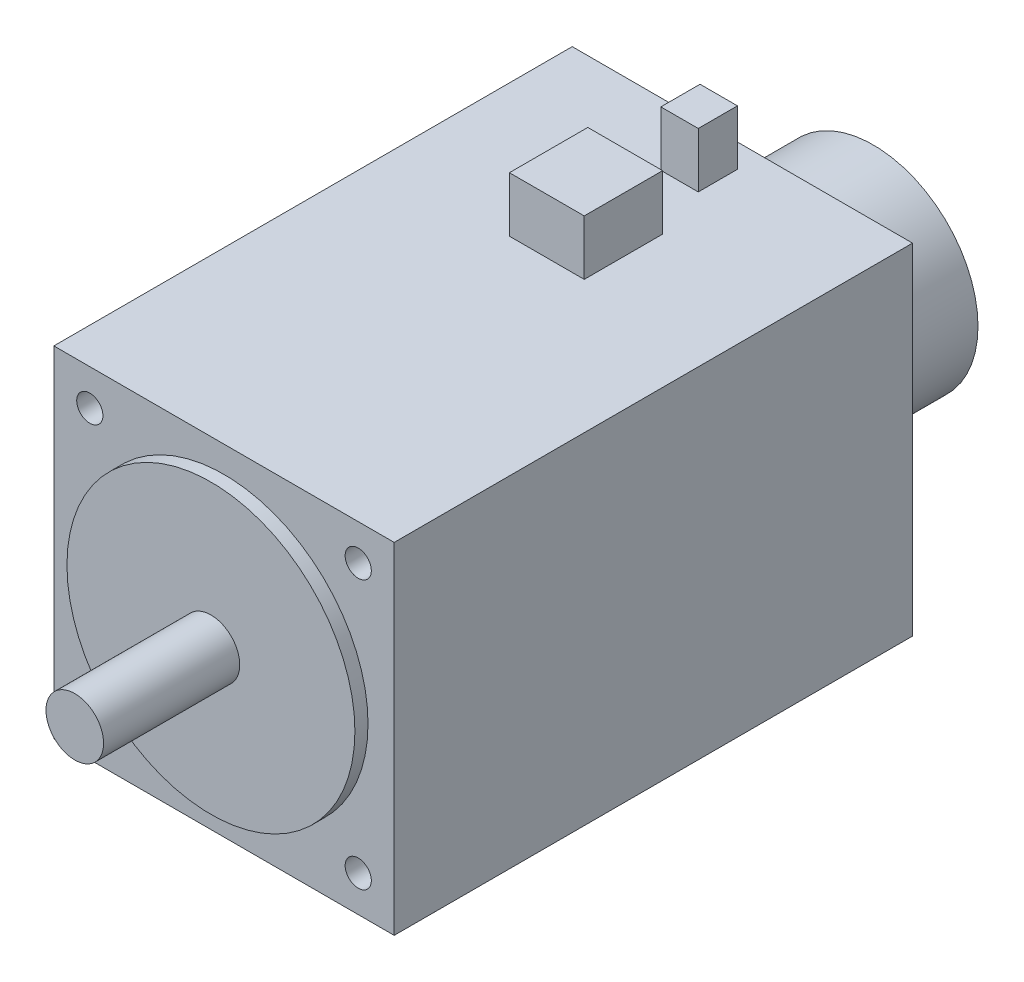
from build123d import *

# Parameters (mm, degrees)
SKETCH_1_W      = 130
SKETCH_1_H      = 130
SKETCH_1_R      = 5
EXTRUDE_1_DEPTH = 99
SKETCH_2_R      = 55
EXTRUDE_2_DEPTH = 5
SKETCH_3_R      = 11
EXTRUDE_3_DEPTH = 52
SKETCH_5_W      = 28.58431815
SKETCH_5_H      = 29.945476157
SKETCH_5_W_2    = 14.292159074
SKETCH_5_H_2    = 14.972738078
EXTRUDE_4_DEPTH = 86
SKETCH_6_R      = 40
EXTRUDE_5_DEPTH = 50


with BuildPart() as part:
    # 草图1 → 凸台-拉伸1 (new, symmetric)
    with BuildSketch(Plane.XY):
        Rectangle(SKETCH_1_W, SKETCH_1_H)
        with Locations((-51.265241636, 51.265241636)):
            Circle(SKETCH_1_R, mode=Mode.SUBTRACT)
        with Locations(Location((51.265241636, 51.265241636, 0), (0, 0, 180))):
            Circle(SKETCH_1_R, mode=Mode.SUBTRACT)
        with Locations(Location((-51.265241636, -51.265241636, 0), (0, 0, 180))):
            Circle(SKETCH_1_R, mode=Mode.SUBTRACT)
        with Locations((51.265241636, -51.265241636)):
            Circle(SKETCH_1_R, mode=Mode.SUBTRACT)
    extrude(amount=EXTRUDE_1_DEPTH, both=True)

    # 草图2 → 凸台-拉伸2 (add)
    with BuildSketch(Plane.XY.offset(99)):
        Circle(SKETCH_2_R)
    extrude(amount=EXTRUDE_2_DEPTH)

    # 草图3 → 凸台-拉伸3 (add)
    with BuildSketch(Plane.XY.offset(104)):
        with Locations(Location((0, 0, 0), (0, 0, 180))):
            Circle(SKETCH_3_R)
    extrude(amount=EXTRUDE_3_DEPTH)

    # 草图5 → 凸台-拉伸4 (add)
    with BuildSketch(Plane(origin=(0, 0, 0), x_dir=(1, 0, 0), z_dir=(0, 1, 0))):
        with Locations((0, 39.269782118)):
            Rectangle(SKETCH_5_W, SKETCH_5_H)
        with Locations((0, 82.486548844)):
            Rectangle(SKETCH_5_W_2, SKETCH_5_H_2)
    extrude(amount=EXTRUDE_4_DEPTH)

    # 草图6 → 凸台-拉伸5 (add)
    with BuildSketch(Plane(origin=(0, 0, -99), x_dir=(-1, 0, 0), z_dir=(0, 0, -1))):
        with Locations(Location((0, 0, 0), (0, 0, 180))):
            Circle(SKETCH_6_R)
    extrude(amount=EXTRUDE_5_DEPTH)


solid = part.part
